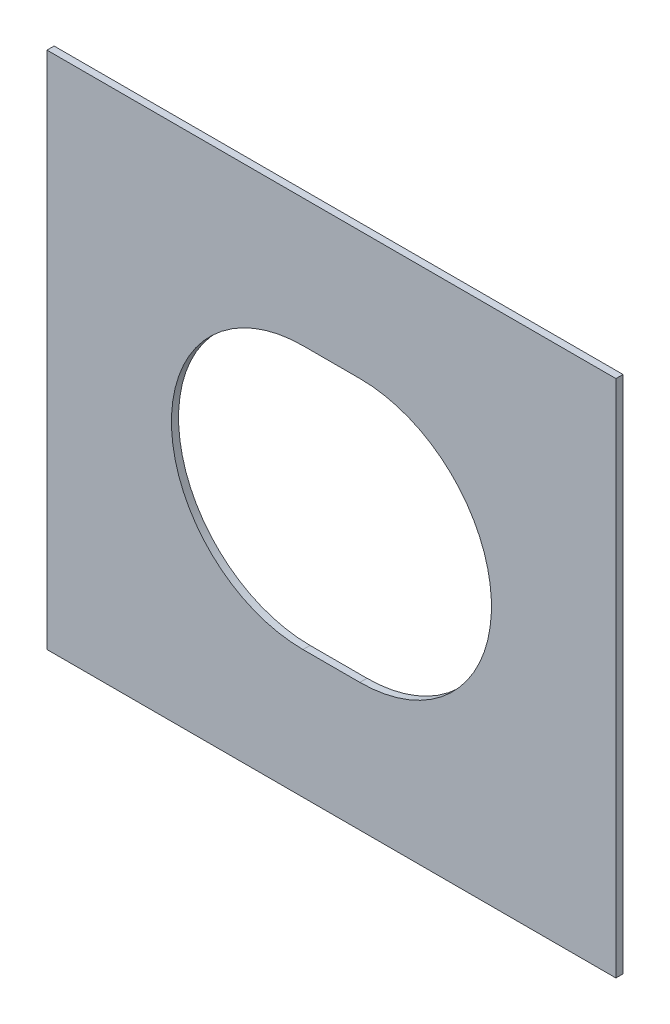
SolidWorks part; units mm, degrees
ref_plane "前视基准面" through (0, 0, 0) normal (0, 0, 1) x (1, 0, 0)
ref_plane "上视基准面" through (0, 0, 0) normal (0, 1, 0) x (1, 0, 0)
ref_plane "右视基准面" through (0, 0, 0) normal (1, 0, 0) x (0, 0, -1)
sketch "草图1" plane through (0, 0, 0) normal (0, 0, 1) x (1, 0, 0)
  line L0 (0, 0) -> (400, 0)
  line L1 (400, 0) -> (400, 365)
  line L2 (400, 365) -> (0, 365)
  line L3 (0, 365) -> (0, 0)
extrude "凸台-拉伸1" add sketch "草图1" along normal blind 5
sketch "草图4" plane through (0, 0, 5) normal (0, 0, 1) x (1, 0, 0)
  line L6 (180, 275) -> (220, 275)
  line L7 (180, 90) -> (220, 90)
  arc A2 (220, 90) -> (220, 275) centre (220, 182.5) ccw
  arc A3 (180, 275) -> (180, 90) centre (180, 182.5) ccw
extrude "切除-拉伸3" cut sketch "草图4" against normal blind 10
